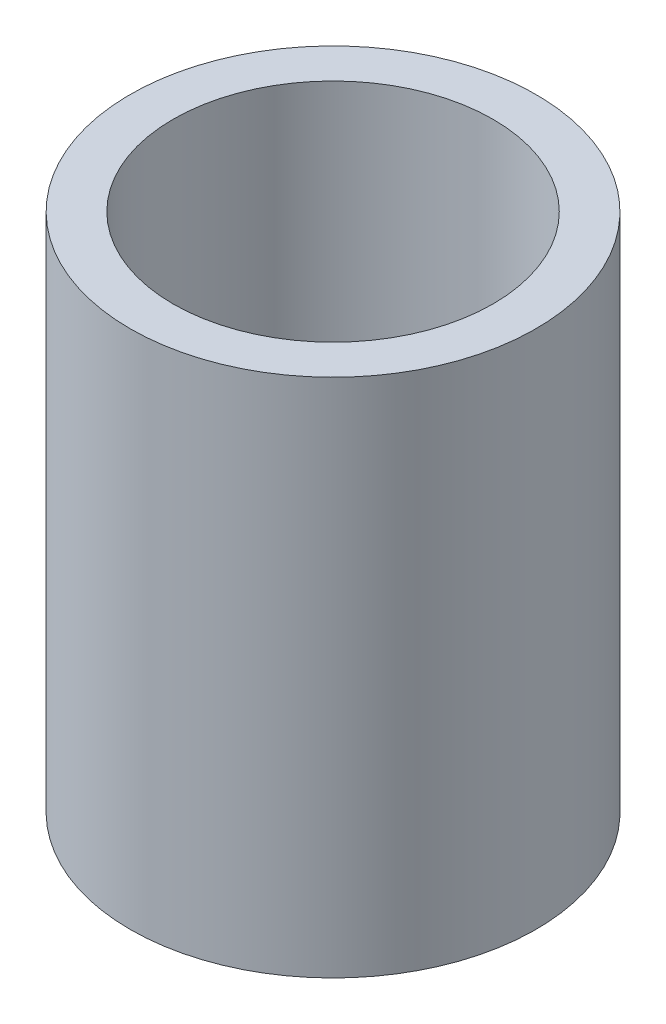
SolidWorks part; units mm, degrees
material "Plain carbon steel"
ref_plane "Front Plane" through (0, 0, 0) normal (0, 0, 1) x (1, 0, 0)
ref_plane "Top Plane" through (0, 0, 0) normal (0, 1, 0) x (1, 0, 0)
ref_plane "Right Plane" through (0, 0, 0) normal (1, 0, 0) x (0, 0, -1)
sketch "Sketch1" plane through (0, 0, 0) normal (0, 1, 0) x (1, 0, 0)
  circle A0 centre (0, 0) radius 19.5
  dimension "D1" = 39
extrude "Boss-Extrude1" add sketch "Sketch1" along normal blind 50
hole_wizard "G1 Tapped Hole1" positions "3DSketch1" profile "Sketch2" tap size "G1" standard "GB" end condition through all
sketch3d "3DSketch1"
  line L0 (0, 50, 0) -> (0, 0, 0) construction
  point P0 (0, 50, 0)
sketch "Sketch2" plane through (0, 50, 0) normal (1, 0, 0) x (0, 0, 1)
  line L0 (0, 0) -> (0, 50)
  line L1 (0, 50) -> (15.375, 50)
  line L2 (15.375, 50) -> (15.375, 0)
  line L5 (15.375, 0) -> (0, 0)
  line L11 (0, -6.35) -> (0, 107.95) construction
  dimension "通孔螺纹孔钻头直径" = 30.75
  dimension "通孔螺纹孔钻头深度" = 50
cosmetic thread "Hole thread1"
